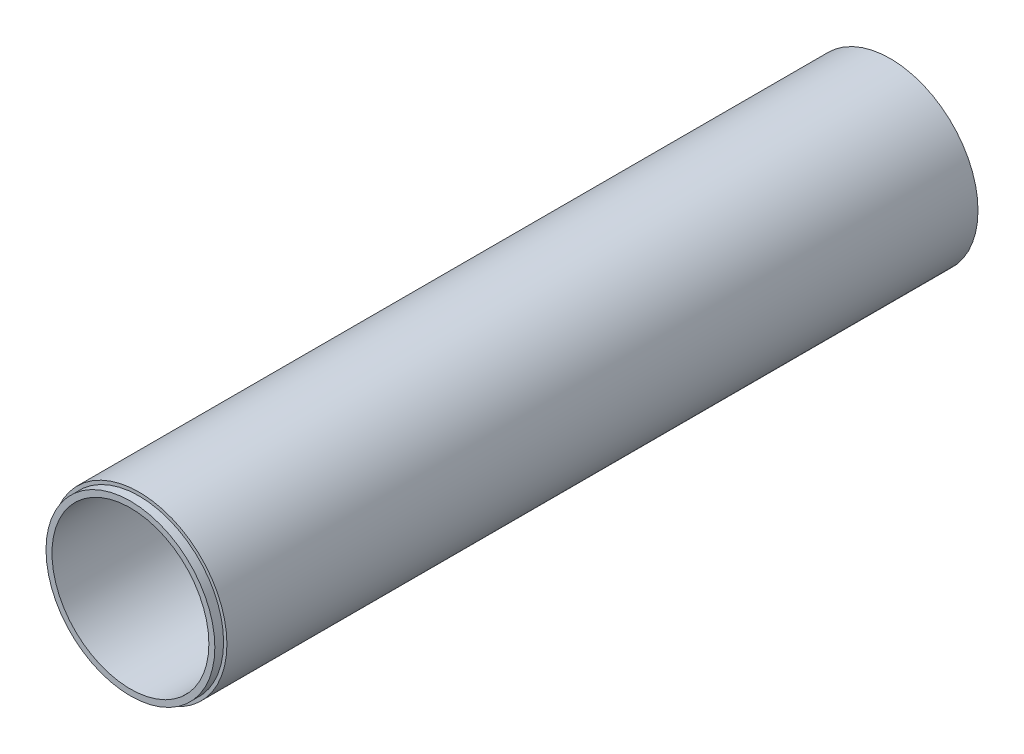
from build123d import *

# Parameters (mm, degrees)
SKETCH_1_R          = 30.15
EXTRUDE_1_DEPTH     = 261
SHELL_1_T           = -3.2
SKETCH_2_OUTSIDE_W  = 117.216
SKETCH_2_OUTSIDE_H  = 117.216
SKETCH_2_OUTSIDE_R  = 29
CUT_EXTRUDE_1_DEPTH = 3


with BuildPart() as part:
    # 草图1 → 凸台-拉伸1 (new body)
    with BuildSketch(Plane.XY):
        Circle(SKETCH_1_R)
    extrude(amount=EXTRUDE_1_DEPTH)

    # 抽壳1
    shell_1_openings = [part.faces().sort_by_distance(p)[0] for p in [
        (0, 0, 261),
        (0, 0, 0),
    ]]
    offset(amount=SHELL_1_T, openings=shell_1_openings, kind=Kind.INTERSECTION)

    # 草图2 outside → 切除-拉伸1 (cut)
    with BuildSketch(Plane.XY.offset(261)):
        Rectangle(SKETCH_2_OUTSIDE_W, SKETCH_2_OUTSIDE_H)
        Circle(SKETCH_2_OUTSIDE_R, mode=Mode.SUBTRACT)
    extrude(amount=-CUT_EXTRUDE_1_DEPTH, mode=Mode.SUBTRACT)


solid = part.part
